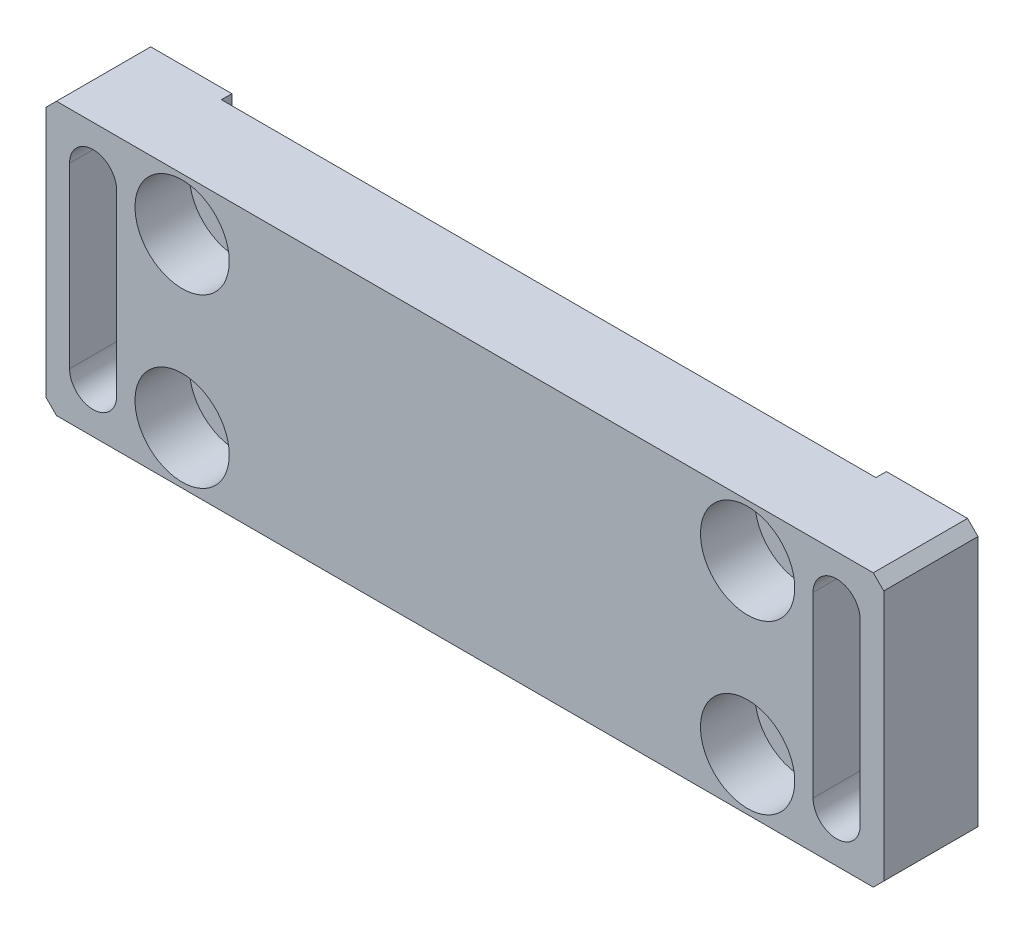
from build123d import *

# Parameters (mm, degrees)
SKETCH1_W           = 80
SKETCH1_H           = 26
BOSS_EXTRUDE1_DEPTH = 9
CUT_EXTRUDE1_REACH  = 45.012
SKETCH2_R           = 2.6
SKETCH3_R           = 4.5
CUT_EXTRUDE2_DEPTH  = 5.2
CUT_EXTRUDE3_REACH  = 45.012
SKETCH8_W           = 62.5
SKETCH8_H           = 26
CUT_EXTRUDE5_DEPTH  = 1
CHAMFER1_SIZE       = 1


with BuildPart() as part:
    # Sketch1 → Boss-Extrude1 (new body)
    with BuildSketch(Plane.XY):
        Rectangle(SKETCH1_W, SKETCH1_H)
    extrude(amount=BOSS_EXTRUDE1_DEPTH)

    # Sketch2 → Cut-Extrude1 (cut, up to next)
    with BuildSketch(Plane.XY.offset(9), mode=Mode.PRIVATE) as cut_extrude1_sk1:
        with Locations((-27, -8)):
            Circle(SKETCH2_R)
    cut_extrude1_tool1 = extrude(cut_extrude1_sk1.sketch, amount=-CUT_EXTRUDE1_REACH, mode=Mode.PRIVATE) & part.part
    # Sketch2 → Cut-Extrude1 (cut, up to next)
    with BuildSketch(Plane.XY.offset(9), mode=Mode.PRIVATE) as cut_extrude1_sk2:
        with Locations((-27, 8)):
            Circle(SKETCH2_R)
    cut_extrude1_tool2 = extrude(cut_extrude1_sk2.sketch, amount=-CUT_EXTRUDE1_REACH, mode=Mode.PRIVATE) & part.part
    # Sketch2 → Cut-Extrude1 (cut, up to next)
    with BuildSketch(Plane.XY.offset(9), mode=Mode.PRIVATE) as cut_extrude1_sk3:
        with Locations((27, 8)):
            Circle(SKETCH2_R)
    cut_extrude1_tool3 = extrude(cut_extrude1_sk3.sketch, amount=-CUT_EXTRUDE1_REACH, mode=Mode.PRIVATE) & part.part
    # Sketch2 → Cut-Extrude1 (cut, up to next)
    with BuildSketch(Plane.XY.offset(9), mode=Mode.PRIVATE) as cut_extrude1_sk4:
        with Locations((27, -8)):
            Circle(SKETCH2_R)
    cut_extrude1_tool4 = extrude(cut_extrude1_sk4.sketch, amount=-CUT_EXTRUDE1_REACH, mode=Mode.PRIVATE) & part.part
    add(cut_extrude1_tool1.solids().sort_by_distance((-27, -8, 9))[0], mode=Mode.SUBTRACT)
    add(cut_extrude1_tool2.solids().sort_by_distance((-27, 8, 9))[0], mode=Mode.SUBTRACT)
    add(cut_extrude1_tool3.solids().sort_by_distance((27, 8, 9))[0], mode=Mode.SUBTRACT)
    add(cut_extrude1_tool4.solids().sort_by_distance((27, -8, 9))[0], mode=Mode.SUBTRACT)

    # Sketch3 → Cut-Extrude2 (cut)
    with BuildSketch(Plane.XY.offset(9)):
        with Locations((-27, -8)):
            Circle(SKETCH3_R)
        with Locations((-27, 8)):
            Circle(SKETCH3_R)
        with Locations((27, 8)):
            Circle(SKETCH3_R)
        with Locations((27, -8)):
            Circle(SKETCH3_R)
    extrude(amount=-CUT_EXTRUDE2_DEPTH, mode=Mode.SUBTRACT)

    # Sketch6 → Cut-Extrude3 (cut, up to next)
    with BuildSketch(Plane(origin=(0, 0, 0), x_dir=(-1, 0, 0), z_dir=(0, 0, -1)), mode=Mode.PRIVATE) as cut_extrude3_sk1:
        with BuildLine():
            Line((-33.25, 8.5), (-33.25, -8.5))
            ThreePointArc((-33.25, -8.5), (-35.5, -10.75), (-37.75, -8.5))
            Line((-37.75, -8.5), (-37.75, 8.5))
            ThreePointArc((-37.75, 8.5), (-35.5, 10.75), (-33.25, 8.5))
        make_face()
    cut_extrude3_tool1 = extrude(cut_extrude3_sk1.sketch, amount=-CUT_EXTRUDE3_REACH, mode=Mode.PRIVATE) & part.part
    cut_extrude3 = cut_extrude3_tool1.solids().sort_by_distance((35.5, 0, 0))[0]
    add(cut_extrude3, mode=Mode.SUBTRACT)

    # Mirror1: Cut-Extrude3 across plane
    add(cut_extrude3.mirror(Plane(origin=(0, 0, 0), x_dir=(0, 0, 1), z_dir=(1, 0, 0))), mode=Mode.SUBTRACT)

    # Sketch8 → Cut-Extrude5 (cut)
    with BuildSketch(Plane(origin=(0, 0, 0), x_dir=(-1, 0, 0), z_dir=(0, 0, -1))):
        Rectangle(SKETCH8_W, SKETCH8_H)
    extrude(amount=-CUT_EXTRUDE5_DEPTH, mode=Mode.SUBTRACT)

    # Chamfer1
    chamfer1_edges = [part.edges().sort_by_distance(p)[0] for p in [
        (40, -13, 4.5),
        (-40, -13, 4.5),
        (-40, 13, 4.5),
        (40, 13, 4.5),
    ]]
    chamfer(chamfer1_edges, length=CHAMFER1_SIZE)


solid = part.part
